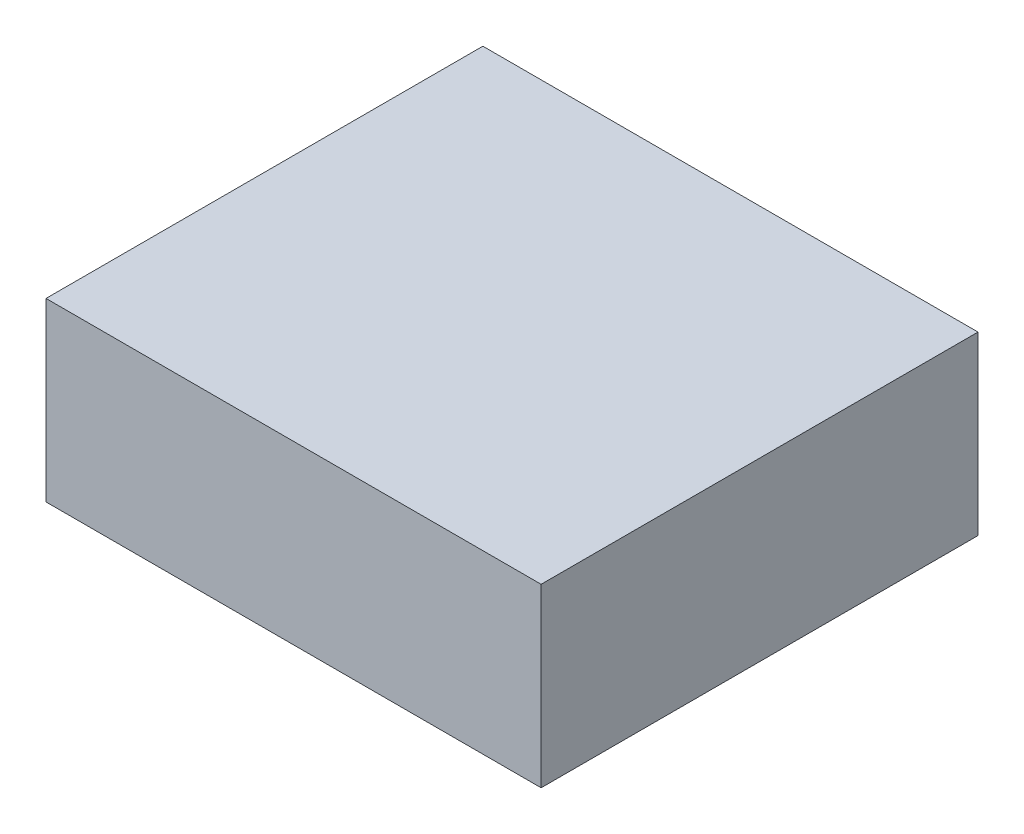
SolidWorks part; units mm, degrees
ref_plane "前视基准面" through (0, 0, 0) normal (0, 0, 1) x (1, 0, 0)
ref_plane "上视基准面" through (0, 0, 0) normal (0, 1, 0) x (1, 0, 0)
ref_plane "右视基准面" through (0, 0, 0) normal (1, 0, 0) x (0, 0, -1)
sketch "草图1" plane through (0, 0, 0) normal (0, 0, 1) x (1, 0, 0)
  line L1 (-117.5163, 35.2207) -> (52.4837, 35.2207)
  line L2 (-117.5163, 35.2207) -> (-117.5163, -25.2993)
  line L3 (-117.5163, -25.2993) -> (52.4837, -25.2993)
  line L4 (52.4837, 35.2207) -> (52.4837, -25.2993)
  dimension "D1" = 60.52
  dimension "D2" = 170
extrude "凸台-拉伸1" add sketch "草图1" along normal blind 150
sketch "草图2" plane through (0, -25.2993, 0) normal (0, -1, 0) x (1, 0, 0)
  line L0 (-117.5163, 150) -> (-117.5163, 0) construction
  line L1 (-107.5163, 140) -> (42.4837, 140)
  line L2 (-107.5163, 140) -> (-107.5163, 10)
  line L3 (-107.5163, 10) -> (42.4837, 10)
  line L4 (42.4837, 140) -> (42.4837, 10)
  line L5 (-117.5163, 150) -> (52.4837, 150) construction
  line L6 (52.4837, 150) -> (52.4837, 0) construction
  line L7 (-117.5163, 0) -> (52.4837, 0) construction
  dimension "D1" = 10
  dimension "D2" = 10
  dimension "D3" = 10
  dimension "D4" = 10
extrude "切除-拉伸1" cut sketch "草图2" against normal blind 50.52
